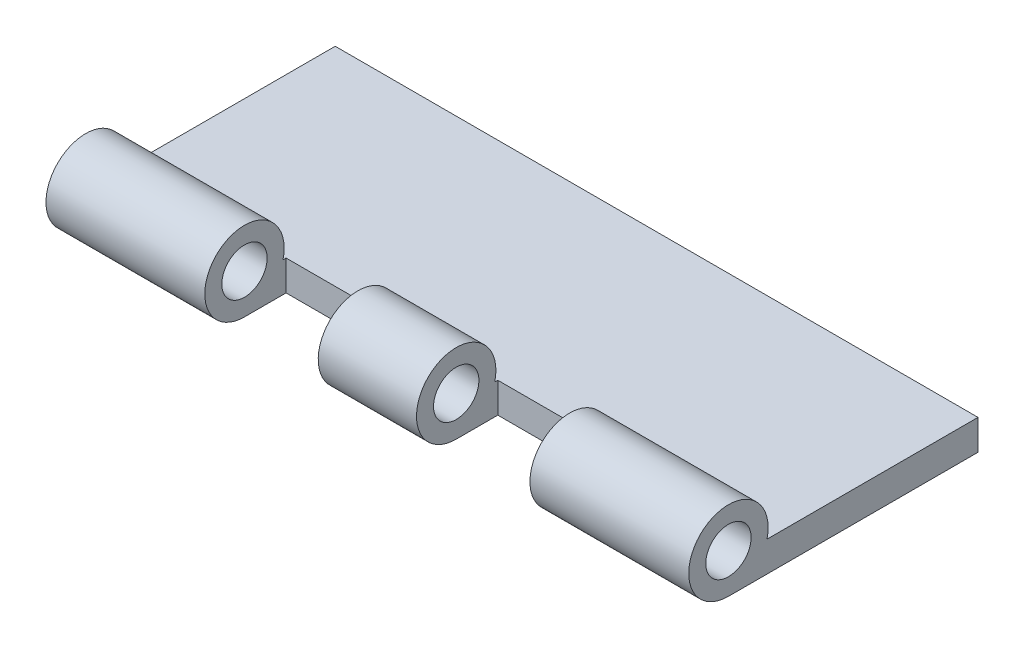
SolidWorks part; units mm, degrees
ref_plane "Front Plane" through (0, 0, 0) normal (0, 0, 1) x (1, 0, 0)
ref_plane "Top Plane" through (0, 0, 0) normal (0, 1, 0) x (1, 0, 0)
ref_plane "Right Plane" through (0, 0, 0) normal (1, 0, 0) x (0, 0, -1)
sketch "Sketch1" plane through (0, 0, 0) normal (1, 0, 0) x (0, 0, -1)
  line L0 (0, 0) -> (14.8083, 0) construction
  line L6 (5.099, -1.25) -> (33, -1.25)
  line L8 (0, -5.25) -> (33, -5.25)
  line L9 (33, -1.25) -> (33, -5.25)
  arc A0 (5.099, -1.25) -> (0, -5.25) centre (0, 0) ccw
  dimension "D1" = 10.5
  dimension "D2" = 4
  dimension "D3" = 33
extrude "Boss-Extrude1" add sketch "Sketch1" along normal mid plane 85
sketch "Sketch2" plane through (0, -1.25, 0) normal (0, 1, 0) x (1, 0, 0)
  line L0 (0, 0) -> (0, 15) construction
  line L1 (-28, 15) -> (28, 15) construction
  circle A0 centre (-28, 15) radius 3
  circle A1 centre (0, 15) radius 3
  circle A2 centre (28, 15) radius 3
  dimension "D2" = 6
  dimension "D1" = 56
  dimension "D3" = 15
extrude "Cut-Extrude1" [suppressed] cut sketch "Sketch2" against normal mid plane 10
chamfer "Chamfer1" [suppressed] distance 4 angle 45
sketch "Sketch3" plane through (0, 0, 0) normal (0, 1, 0) x (1, 0, 0)
  line L0 (0, 0) -> (42.5, 0) construction
  line L2 (42.5, -5.25) -> (42.5, 5.25) construction
  line L3 (0, 0) -> (0, 29.1462) construction
  line L4 (6.5, -5.5) -> (21.5, -5.5)
  line L5 (6.5, -5.5) -> (6.5, 5.5)
  line L6 (6.5, 5.5) -> (21.5, 5.5)
  line L7 (21.5, -5.5) -> (21.5, 5.5)
  line L8 (6.5, -5.5) -> (21.5, 5.5) construction
  line L9 (6.5, 5.5) -> (21.5, -5.5) construction
  line L10 (-6.5, 5.5) -> (-21.5, -5.5) construction
  line L11 (-6.5, -5.5) -> (-21.5, 5.5) construction
  line L12 (-21.5, -5.5) -> (-21.5, 5.5)
  line L13 (-6.5, 5.5) -> (-21.5, 5.5)
  line L14 (-6.5, -5.5) -> (-6.5, 5.5)
  line L15 (-6.5, -5.5) -> (-21.5, -5.5)
  point P7 (14, 0)
  point P15 (-14, 0)
  dimension "D1" = 15
  dimension "D2" = 11
  dimension "D3" = 6.5
extrude "Cut-Extrude2" cut sketch "Sketch3" against normal mid plane 20
sketch "Sketch4" plane through (42.5, 0, 0) normal (1, 0, 0) x (0, 0, -1)
  circle A0 centre (0, 0) radius 3
  dimension "D1" = 6
extrude "Cut-Extrude3" cut sketch "Sketch4" against normal through all
